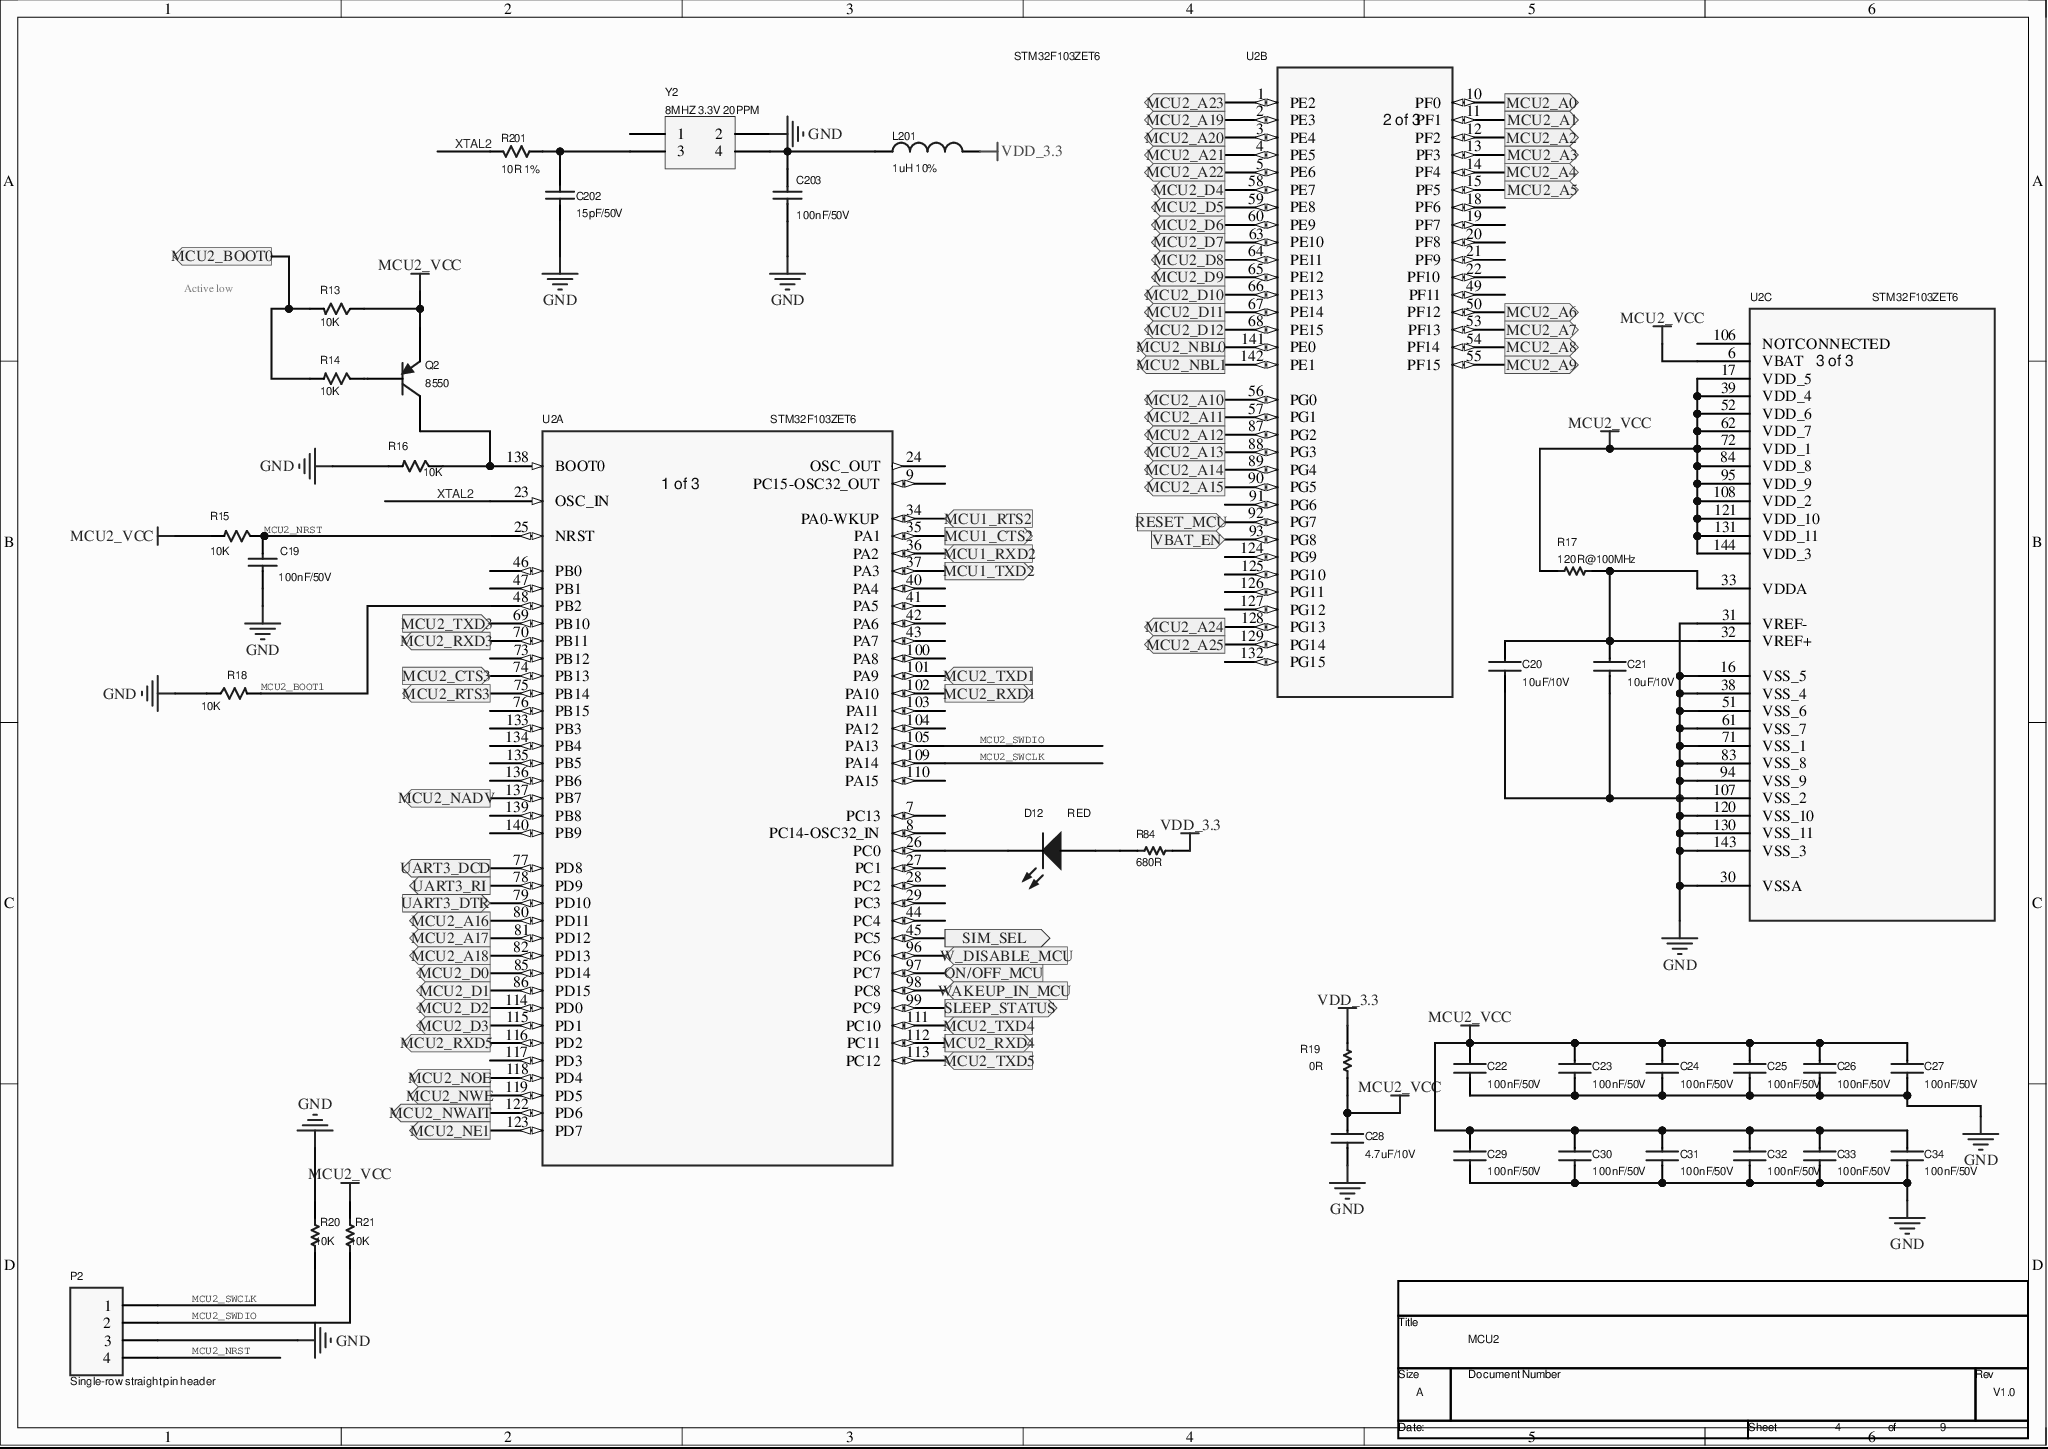
[diagram p0: MISC86294-8.SchDoc]
# Altium project MISC86294-22.PrjPcb (part 2 of 5)

## Sheet MISC86294-8.SchDoc
size 297 x 209 mm

### Parts
(Parts that share a designator on the sheet are numbered #1, #2 ... from top to bottom, then left to right.)
*#4  RevCode: V1.0  Title: MCU2  Page Size: A  Page Number: 4  Page Count: 9  (hidden comment: TitleBlock0)  (graphical)
C19  100nF/50V  [0603]
C20  10uF/10V  [C0603]
C21  10uF/10V  [C0603]
C22  100nF/50V  [C0603]
C23  100nF/50V  [C0603]
C24  100nF/50V  [C0603]
C25  100nF/50V  [C0603]
C26  100nF/50V  [C0603]
C27  100nF/50V  [C0603]
C28  4.7uF/10V  [C0805]
C29  100nF/50V  [C0603]
C30  100nF/50V  [C0603]
C31  100nF/50V  [C0603]
C32  100nF/50V  [C0603]
C33  100nF/50V  [C0603]
C34  100nF/50V  [C0603]
C202  15pF/50V  [C0603]
C203  100nF/50V  [C0603]
D12  RED  [LED_0805]
L201  1uH 10%  [SMD_L6.0-W6.0]
P2  Single-row straight pin header  [HDR1X4]
Q2  8550  [SOT-23-SS8550]
R13  10K  [0603]
R14  10K  [0603]
R15  10K  [0603]
R16  10K  [0603]
R17  120R@100MHz  [0603]
R18  10K  [0603]
R19  0R  [0603]
R20  10K  [0603]
R21  10K  [0603]
R84  User_Value: 680R  [0603]  (hidden comment: NA)
R201  10R 1%  [R0805]
U2  STM32F103ZET6  [LQFP144-20x20mm]  (parts A,B,C of 3)
Y2  8MHZ 3.3V 20PPM  [XTAL 5.7X7.0-SM - duplicate]

### Ports
MCU1_CTS2 (out), MCU1_RTS2 (in), MCU1_RXD2 (in), MCU1_TXD2 (out), MCU2_A0 (out), MCU2_A1 (out), MCU2_A2 (out), MCU2_A3 (out), MCU2_A4 (out), MCU2_A5 (out), MCU2_A6 (out), MCU2_A7 (out), MCU2_A8 (out), MCU2_A9 (out), MCU2_A10 (out), MCU2_A11 (out), MCU2_A12 (out), MCU2_A13 (out), MCU2_A14 (out), MCU2_A15 (out), MCU2_A16 (out), MCU2_A17 (out), MCU2_A18 (out), MCU2_A19 (out), MCU2_A20 (out), MCU2_A21 (out), MCU2_A22 (out), MCU2_A23 (out), MCU2_A24 (out), MCU2_A25 (out), MCU2_BOOT0 (out), MCU2_CTS3 (in), MCU2_D0 (out), MCU2_D1 (out), MCU2_D2 (out), MCU2_D3 (out), MCU2_D4 (out), MCU2_D5 (out), MCU2_D6 (out), MCU2_D7 (out), MCU2_D8 (out), MCU2_D9 (out), MCU2_D10 (out), MCU2_D11 (out), MCU2_D12 (out), MCU2_NADV (out), MCU2_NBL0 (out), MCU2_NBL1 (out), MCU2_NE1 (out), MCU2_NOE (out), MCU2_NWAIT (out), MCU2_NWE (out), MCU2_RTS3 (out), MCU2_RXD1 (out), MCU2_RXD3 (out), MCU2_RXD4 (out), MCU2_RXD5 (out), MCU2_TXD1 (in), MCU2_TXD3 (in), MCU2_TXD4 (in), MCU2_TXD5 (in), ON/OFF_MCU (in), RESET_MCU (in), SIM_SEL (out), SLEEP_STATUS (out), UART3_DCD (out), UART3_DTR (in), UART3_RI (out), VBAT_EN (in), W_DISABLE_MCU (in), WAKEUP_IN_MCU (in)

### Nets
GND: C19.1 C20.2 C21.2 C22.2 C23.2 C24.2 C25.2 C26.2 C27.2 C28.2 C29.2 C30.2 C31.2 C32.2 C33.2 C34.2 C202.1 C203.2 P2.3 R16.1 R18.1 R20.2 U2.16(VSS_5) U2.30(VSSA) U2.31(VREF-) U2.38(VSS_4) U2.51(VSS_6) U2.61(VSS_7) U2.71(VSS_1) U2.83(VSS_8) U2.94(VSS_9) U2.107(VSS_2) U2.120(VSS_10) U2.130(VSS_11) U2.143(VSS_3) Y2.2
MCU2_VCC: C22.1 C23.1 C24.1 C25.1 C26.1 C27.1 C28.1 C29.1 C30.1 C31.1 C32.1 C33.1 C34.1 Q2.2(E) R13.2 R15.2 R17.1 R19.2 R21.2 U2.6(VBAT) U2.17(VDD_5) U2.39(VDD_4) U2.52(VDD_6) U2.62(VDD_7) U2.72(VDD_1) U2.84(VDD_8) U2.95(VDD_9) U2.108(VDD_2) U2.121(VDD_10) U2.131(VDD_11) U2.144(VDD_3)
VDD_3.3: L201.2 R19.1 R84.1
MCU2_BOOT1: R18.2 U2.48(PB2)
MCU2_NRST: C19.2 P2.4 R15.1 U2.25(NRST)
MCU2_SWCLK: P2.1 R20.1 U2.109(PA14)
MCU2_SWDIO: P2.2 R21.1 U2.105(PA13)
XTAL2: R201.1 U2.23(OSC_IN)
NetC20_1: C20.1 C21.1 R17.2 U2.32(VREF+) U2.33(VDDA)
NetC202_2: C202.2 R201.2 Y2.3
NetC203_1: C203.1 L201.1 Y2.4
NetD12_1: D12.1(A) R84.2
NetD12_2: D12.2(K) U2.26(PC0)
NetJ6_37: U2.102(PA10) ; port MCU2_RXD1
NetJ6_38: U2.101(PA9) ; port MCU2_TXD1
NetJ14_1: U2.37(PA3) ; port MCU1_TXD2
NetJ14_2: U2.36(PA2) ; port MCU1_RXD2
NetJ17_1: U2.69(PB10) ; port MCU2_TXD3
NetJ17_2: U2.70(PB11) ; port MCU2_RXD3
NetJ19_1: U2.111(PC10) ; port MCU2_TXD4
NetJ19_2: U2.112(PC11) ; port MCU2_RXD4
NetJ21_1: U2.113(PC12) ; port MCU2_TXD5
NetJ21_2: U2.116(PD2) ; port MCU2_RXD5
NetJ23_1: U2.45(PC5) ; port SIM_SEL
NetP3_12: R13.1 R14.2 ; port MCU2_BOOT0
NetQ2_1: Q2.1(B) R14.1
NetQ2_3: Q2.3(C) R16.2 U2.138(BOOT0)
NetQ3_1: U2.74(PB13) ; port MCU2_CTS3
NetQ5_1: U2.79(PD10) ; port UART3_DTR
NetQ6_3: U2.75(PB14) ; port MCU2_RTS3
NetQ8_3: U2.77(PD8) ; port UART3_DCD
NetQ9_3: U2.78(PD9) ; port UART3_RI
NetQ10_1: U2.99(PC9) ; port SLEEP_STATUS
NetQ11_1: U2.93(PG8) ; port VBAT_EN
NetQ12_1: U2.96(PC6) ; port W_DISABLE_MCU
NetQ13_1: U2.92(PG7) ; port RESET_MCU
NetQ14_1: U2.97(PC7) ; port ON/OFF_MCU
NetQ17_1: U2.98(PC8) ; port WAKEUP_IN_MCU
NetU1_34: U2.35(PA1) ; port MCU1_CTS2
NetU1_35: U2.34(PA0-WKUP) ; port MCU1_RTS2
NetU2_1: U2.1(PE2) ; port MCU2_A23
NetU2_2: U2.2(PE3) ; port MCU2_A19
NetU2_3: U2.3(PE4) ; port MCU2_A20
NetU2_4: U2.4(PE5) ; port MCU2_A21
NetU2_5: U2.5(PE6) ; port MCU2_A22
NetU2_10: U2.10(PF0) ; port MCU2_A0
NetU2_11: U2.11(PF1) ; port MCU2_A1
NetU2_12: U2.12(PF2) ; port MCU2_A2
NetU2_13: U2.13(PF3) ; port MCU2_A3
NetU2_14: U2.14(PF4) ; port MCU2_A4
NetU2_15: U2.15(PF5) ; port MCU2_A5
NetU2_50: U2.50(PF12) ; port MCU2_A6
NetU2_53: U2.53(PF13) ; port MCU2_A7
NetU2_54: U2.54(PF14) ; port MCU2_A8
NetU2_55: U2.55(PF15) ; port MCU2_A9
NetU2_56: U2.56(PG0) ; port MCU2_A10
NetU2_57: U2.57(PG1) ; port MCU2_A11
NetU2_58: U2.58(PE7) ; port MCU2_D4
NetU2_59: U2.59(PE8) ; port MCU2_D5
NetU2_60: U2.60(PE9) ; port MCU2_D6
NetU2_63: U2.63(PE10) ; port MCU2_D7
NetU2_64: U2.64(PE11) ; port MCU2_D8
NetU2_65: U2.65(PE12) ; port MCU2_D9
NetU2_66: U2.66(PE13) ; port MCU2_D10
NetU2_67: U2.67(PE14) ; port MCU2_D11
NetU2_68: U2.68(PE15) ; port MCU2_D12
NetU2_80: U2.80(PD11) ; port MCU2_A16
NetU2_81: U2.81(PD12) ; port MCU2_A17
NetU2_82: U2.82(PD13) ; port MCU2_A18
NetU2_85: U2.85(PD14) ; port MCU2_D0
NetU2_86: U2.86(PD15) ; port MCU2_D1
NetU2_87: U2.87(PG2) ; port MCU2_A12
NetU2_88: U2.88(PG3) ; port MCU2_A13
NetU2_89: U2.89(PG4) ; port MCU2_A14
NetU2_90: U2.90(PG5) ; port MCU2_A15
NetU2_114: U2.114(PD0) ; port MCU2_D2
NetU2_115: U2.115(PD1) ; port MCU2_D3
NetU2_118: U2.118(PD4) ; port MCU2_NOE
NetU2_119: U2.119(PD5) ; port MCU2_NWE
NetU2_122: U2.122(PD6) ; port MCU2_NWAIT
NetU2_123: U2.123(PD7) ; port MCU2_NE1
NetU2_128: U2.128(PG13) ; port MCU2_A24
NetU2_129: U2.129(PG14) ; port MCU2_A25
NetU2_137: U2.137(PB7) ; port MCU2_NADV
NetU2_141: U2.141(PE0) ; port MCU2_NBL0
NetU2_142: U2.142(PE1) ; port MCU2_NBL1

Not connected (* = marked no-connect by the designer): U2 7(PC13) 8(PC14-OSC32_IN) 9(PC15-OSC32_OUT) 18(PF6) 19(PF7) 20(PF8) 21(PF9) 22(PF10) 24(OSC_OUT) 27(PC1) 28(PC2) 29(PC3) 40(PA4) 41(PA5) 42(PA6) 43(PA7) 44(PC4) 46(PB0) 47(PB1) 49(PF11) 73(PB12) 76(PB15) 91(PG6) 100(PA8) 103(PA11) 104(PA12) 106(NOTCONNECTED) 110(PA15) 117(PD3) 124(PG9) 125(PG10) 126(PG11) 127(PG12) 132(PG15) 133(PB3) 134(PB4) 135(PB5) 136(PB6) 139(PB8) 140(PB9); Y2 1

### Notes on the sheet
- Active low

### Library data of the parts
*#4 = TitleBlock0: Document: Agr-Ctrl-3GS-04; Page Create Date: March  8, 1995
C19 = Cap_C14: Kind: General; SubKind: Capacitor; Origin: Altium; Published: 8-Jun-2000; Revision: July-2002: Re-released for DXP Platform.; User_Value: 100nF/50V; Spice Prefix: C; Type: Capacitor; Publisher: Altium Limited
C20-C34 = CAP NP_Dup1
C202 C203 = Cap: SMD capacitor; Published: 8-Jun-2000; Revision: July-2002: Re-released for DXP Platform.; Publisher: Altium Limited
  C202: Value: 15pF/50V
  C203: Value: 100nF/50V
D12 = LED1_D4: Kind: General; SubKind: Diode; Origin: Altium; Published: 8-Jun-2000; LatestRevisionDate: 08-Jul-2005; LatestRevisionNote: Mech Layer 1 removed.; PackageReference: LED-1; Spice Prefix: D; Publisher: Altium Limited
L201 = Inductor: SMD inductor; Code_IEC: 1005; Published: 8-Jun-2000; LatestRevisionDate: 17-Jul-2002; LatestRevisionNote: Re-released for DXP Platform.; PackageReference: 0402-A; Code_JEITA: 0402; Value: 1uH 10%; Publisher: Altium Limited
P2 = Header 4_P1: Origin: Altium; LatestRevisionDate: 17-Jul-2002; LatestRevisionNote: Re-released for DXP Platform.; Type: Connector; Publisher: Altium Limited
Q2 = PNP_Q1: Kind: Transistor; SubKind: BJT; Origin: Altium; Published: 8-Jun-2000; LatestRevisionDate: 29-May-2009; LatestRevisionNote: IPC-7351 Footprint Added.; PackageVersion: Aug-1999; PackageReference: SOT-23B; PackageDescription: 3-Pin SOT-23 Package 0.95 mm Pitch, 2.4 mm Lead Span; Created: 5/07/2006; Spice Prefix: Q; Type: BJT; Publisher: Altium Limited
R13 = Res_R2: Kind: General; SubKind: Resistor; Origin: Altium; Published: 8-Jun-2000; LatestRevisionDate: 04-Mar-2005; LatestRevisionNote: PCB Footprint replaced.; PackageReference: J1-0603; User_Value: 10K; Spice Prefix: R; Type: Resistor; Publisher: Altium Limited
R14 = Res_R3: Kind: General; SubKind: Resistor; Origin: Altium; Published: 8-Jun-2000; LatestRevisionDate: 04-Mar-2005; LatestRevisionNote: PCB Footprint replaced.; PackageReference: J1-0603; User_Value: 10K; Spice Prefix: R; Type: Resistor; Publisher: Altium Limited
R15 = Res_R5: Kind: General; SubKind: Resistor; Origin: Altium; Published: 8-Jun-2000; LatestRevisionDate: 04-Mar-2005; LatestRevisionNote: PCB Footprint replaced.; PackageReference: J1-0603; User_Value: 10K; Spice Prefix: R; Type: Resistor; Publisher: Altium Limited
R16 = Res_R4: Kind: General; SubKind: Resistor; Origin: Altium; Published: 8-Jun-2000; LatestRevisionDate: 04-Mar-2005; LatestRevisionNote: PCB Footprint replaced.; PackageReference: J1-0603; User_Value: 10K; Spice Prefix: R; Type: Resistor; Publisher: Altium Limited
R17 R19 = Res1_R21: Kind: General; SubKind: Resistor; Origin: Altium; Published: 8-Jun-2000; LatestRevisionDate: 17-Jul-2002; LatestRevisionNote: Re-released for DXP Platform.; PackageReference: AXIAL-0.3; Spice Prefix: R; Type: Resistor; Publisher: Altium Limited
  R17: User_Value: 120R@100MHz
  R19: User_Value: 0R
R18 = Res_R1: Kind: General; SubKind: Resistor; Origin: Altium; Published: 8-Jun-2000; LatestRevisionDate: 04-Mar-2005; LatestRevisionNote: PCB Footprint replaced.; PackageReference: J1-0603; User_Value: 10K; Spice Prefix: R; Type: Resistor; Publisher: Altium Limited
R20 = Res1_R6: Kind: General; SubKind: Resistor; Origin: Altium; Published: 8-Jun-2000; LatestRevisionDate: 17-Jul-2002; LatestRevisionNote: Re-released for DXP Platform.; PackageReference: AXIAL-0.3; User_Value: 10K; Spice Prefix: R; Type: Resistor; Publisher: Altium Limited
R21 = Res1_R7: Kind: General; SubKind: Resistor; Origin: Altium; Published: 8-Jun-2000; LatestRevisionDate: 17-Jul-2002; LatestRevisionNote: Re-released for DXP Platform.; PackageReference: AXIAL-0.3; User_Value: 10K; Spice Prefix: R; Type: Resistor; Publisher: Altium Limited
R84 = Res1_R8: Origin: Altium; Published: 8-Jun-2000; LatestRevisionDate: 17-Jul-2002; LatestRevisionNote: Re-released for DXP Platform.; PackageReference: AXIAL-0.3; Publisher: Altium Limited
R201 = Res: SMD resistor; Published: 8-Jun-2000; LatestRevisionDate: 04-Mar-2005; LatestRevisionNote: PCB Footprint replaced.; PackageReference: J1-0603; Value: 10R 1%; Publisher: Altium Limited
U2 = STM32F103ZET6: Mfr_Name: STMicroelectronics; Manufacturer_Part_Number: STM32F103ZET6; Copyright: Copyright (C) 2022 Ultra Librarian. All rights reserved.
Y2 = Header 2X2: Header, 2-Pin, Dual row; LatestRevisionDate: 17-Jul-2002; LatestRevisionNote: Re-released for DXP Platform.; Publisher: Altium Limited

## Sheet MISC86294-10.SchDoc
size 297 x 209 mm